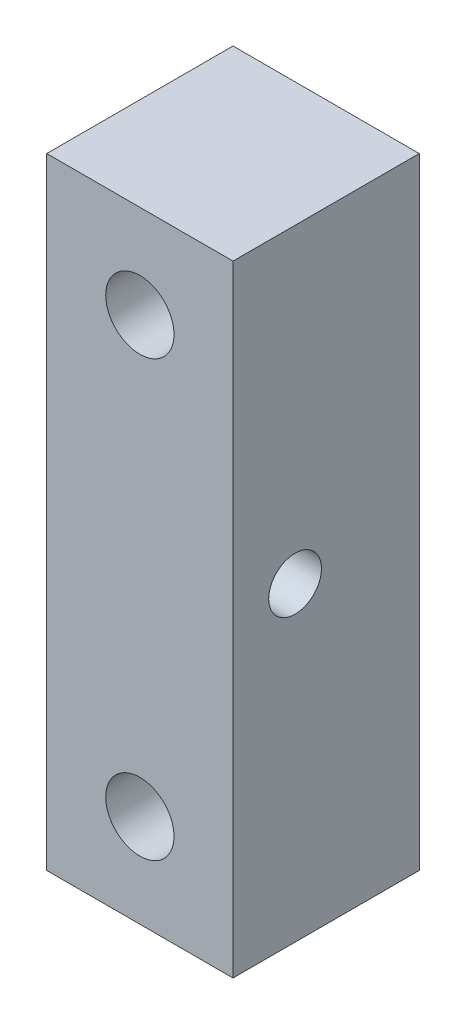
SolidWorks part; units mm, degrees
ref_plane "前视基准面" through (0, 0, 0) normal (0, 0, 1) x (1, 0, 0)
ref_plane "上视基准面" through (0, 0, 0) normal (0, 1, 0) x (1, 0, 0)
ref_plane "右视基准面" through (0, 0, 0) normal (1, 0, 0) x (0, 0, -1)
sketch "草图1" plane through (0, 0, 0) normal (0, 1, 0) x (1, 0, 0)
  line L1 (-15, -15) -> (15, -15)
  line L2 (-15, -15) -> (-15, 15)
  line L3 (-15, 15) -> (15, 15)
  line L4 (15, -15) -> (15, 15)
  line L5 (-15, -15) -> (15, 15) construction
  line L6 (-15, 15) -> (15, -15) construction
  point P0 (0, 0)
  dimension "D1" = 30
  dimension "D2" = 30
extrude "凸台-拉伸1" add sketch "草图1" along normal blind 100
hole_wizard "打孔尺寸(%根据)内六角圆柱头螺钉的类型1" positions "草图2" profile "草图4" counterbore size "M10" standard "GB" end condition through all
sketch "草图2" plane through (0, 0, -15) normal (0, 0, -1) x (-1, 0, 0)
  line L0 (-15, 100) -> (15, 100) construction
  line L1 (-15, 0) -> (15, 0) construction
  point P0 (0, 15)
  point P2 (0, 85)
  dimension "D1" = 15
  dimension "D2" = 15
sketch "草图4" plane through (0, 15, -15) normal (1, 0, 0) x (0, 1, 0)
  line L0 (0, 0) -> (0, 30)
  line L1 (0, 30) -> (5.5, 30)
  line L3 (5.5, 30) -> (5.5, 11)
  line L4 (5.5, 11) -> (9, 11)
  line L5 (9, 11) -> (9, 0)
  line L7 (9, 0) -> (0, 0)
  line L11 (0, -6.35) -> (0, 107.95) construction
  dimension "通孔孔直径" = 11
  dimension "通孔孔深度" = 30
  dimension "柱形沉头孔直径" = 18
  dimension "柱形沉头孔深度" = 11
hole_wizard "M10 螺纹孔1" positions "草图5" profile "草图6" tap size "M10" standard "GB" end condition through all
sketch "草图5" plane through (-15, 0, 0) normal (-1, 0, 0) x (0, 0, 1)
  line L0 (-15, 100) -> (-15, 0) construction
  line L1 (15, 100) -> (15, 0) construction
  point P0 (5, 50)
  point P5 (-15, 50)
  dimension "D1" = 10
sketch "草图6" plane through (-15, 50, 5) normal (0, 1, 0) x (0, 0, 1)
  line L0 (0, 0) -> (0, 30)
  line L1 (0, 30) -> (4.25, 30)
  line L2 (4.25, 30) -> (4.25, 0)
  line L5 (4.25, 0) -> (0, 0)
  line L11 (0, -6.35) -> (0, 107.95) construction
  dimension "通孔螺纹孔钻头直径" = 8.5
  dimension "通孔螺纹孔钻头深度" = 30
cosmetic thread "孔螺蚊线1" parameters "D2"=10
